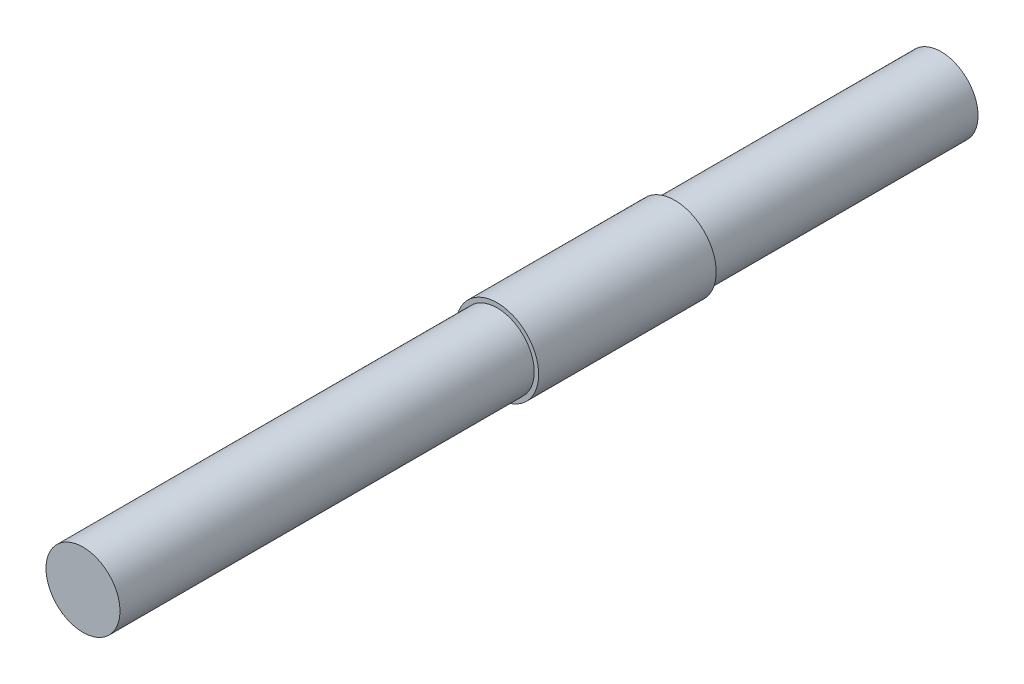
SolidWorks part; units mm, degrees
ref_plane "Front Plane" through (0, 0, 0) normal (0, 0, 1) x (1, 0, 0)
ref_plane "Top Plane" through (0, 0, 0) normal (0, 1, 0) x (1, 0, 0)
ref_plane "Right Plane" through (0, 0, 0) normal (1, 0, 0) x (0, 0, -1)
ref_plane "Plane1" through (0, 889.9765, 0) normal (0, -1, 0) x (1, 0, 0)
sketch "Sketch1" plane through (0, 889.9765, 0) normal (0, -1, 0) x (1, 0, 0)
  line L0 (533.7306, -100.893) -> (521.2306, -100.893)
  line L1 (521.2306, -100.893) -> (521.2306, -390.893)
  line L2 (521.2306, -390.893) -> (533.7306, -390.893)
  line L3 (533.7306, -390.893) -> (533.7306, -300.893)
  line L4 (533.7306, -300.893) -> (535.2306, -300.893)
  line L5 (535.2306, -300.893) -> (535.2306, -240.893)
  line L6 (535.2306, -240.893) -> (533.7306, -240.893)
  line L7 (533.7306, -240.893) -> (533.7306, -100.893)
  line L8 (521.2306, -100.893) -> (521.2306, -390.893) construction
  dimension "D1" = 12.5
  dimension "D2" = 14
  dimension "D3" = 90
  dimension "D4" = 150
  dimension "D5" = 290
revolve "Revolve1" add sketch "Sketch1" angle 360 about L8
sketch "Sketch2" plane through (0, 0, -100.893) normal (0, 0, 1) x (1, 0, 0)
  line L0 (521.2306, 889.9765) -> (508.7306, 889.9765)
  circle A0 centre (521.2306, 889.9765) radius 12.5 construction
sketch "Sketch3" plane through (0, 0, -390.893) normal (0, 0, -1) x (-1, 0, 0)
  line L0 (-521.2306, 889.9765) -> (-508.7306, 889.9765)
  circle A0 centre (-521.2306, 889.9765) radius 12.5 construction
